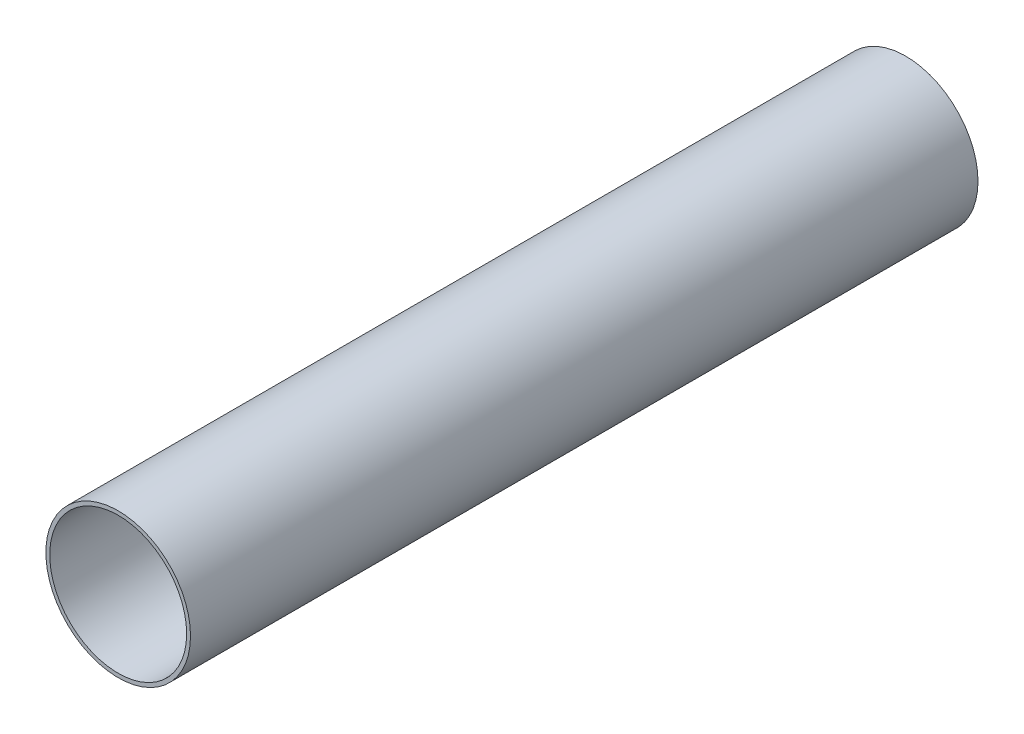
from build123d import *

# Parameters (mm, degrees)
SKETCH1_R           = 22.5
SKETCH1_R_2         = 21.3
BOSS_EXTRUDE1_DEPTH = 245


with BuildPart() as part:
    # Sketch1 → Boss-Extrude1 (new body)
    with BuildSketch(Plane.XY):
        Circle(SKETCH1_R)
        Circle(SKETCH1_R_2, mode=Mode.SUBTRACT)
    extrude(amount=BOSS_EXTRUDE1_DEPTH)


solid = part.part
